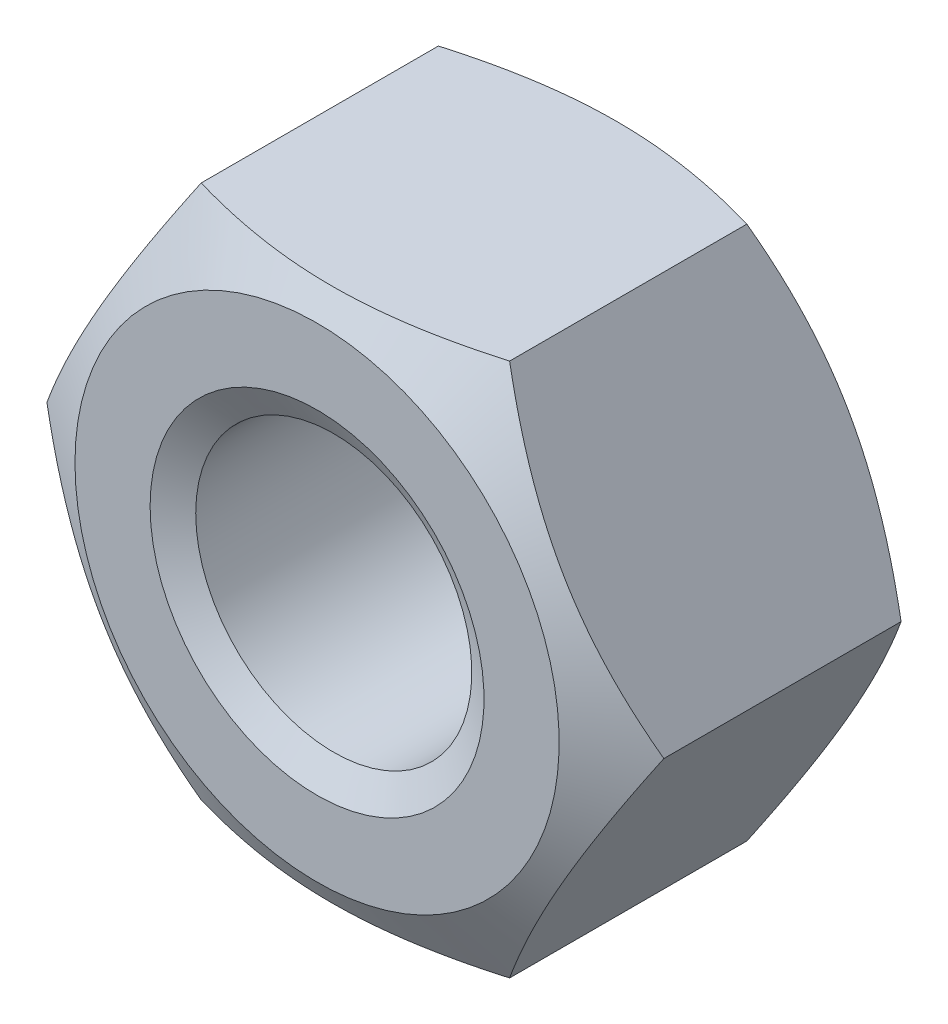
from build123d import *
from OCP.BRepFilletAPI import BRepFilletAPI_MakeChamfer

# Parameters (mm, degrees)
SKETCH1_R        = 2.067
BASENUT_DEPTH    = 4.7
ENDCHAMFER_SIZE  = 0.433
ENDCHAMFER_SIZE2 = 0.249992667


with BuildPart() as part:
    # Sketch1 → BaseNut (new body)
    with BuildSketch(Plane.XY):
        Polygon((4.618802154, 0), (2.309401077, 4), (-2.309401077, 4), (-4.618802154, 0), (-2.309401077, -4), (2.309401077, -4), align=None)
        Circle(SKETCH1_R, mode=Mode.SUBTRACT)
    extrude(amount=-BASENUT_DEPTH)

    # Sketch2 → Double-Chamfer (revolve, cut)
    with BuildSketch(Plane(origin=(0, 0, 0), x_dir=(1, 0, 0), z_dir=(0, 1, 0))):
        Polygon((-4.618802154, 4.7), (-3.625, 4.7), (-4.618802154, 4.126228059), align=None)
        Polygon((-4.618802154, 0.573771941), (-4.618802154, 0), (-3.625, 0), align=None)
    revolve(axis=Axis((0, 0, -3.375940562), (0, 0, 1)), mode=Mode.SUBTRACT)

    # EndChamfer: one chamfer whose edges measure the first distance from different faces: ONE call of the kernel's chamfer builder (chamfer() names one face for all edges)
    endchamfer_edges_1 = [part.edges().sort_by_distance(p)[0] for p in [
        (-2.067, 0, -4.7),
    ]]
    endchamfer_side_1 = [part.faces().sort_by_distance(p)[0] for p in [
        (-2.067, 0, -2.35),
    ]]
    endchamfer_edges_2 = [part.edges().sort_by_distance(p)[0] for p in [
        (-2.067, 0, 0),
    ]]
    endchamfer_side_2 = [part.faces().sort_by_distance(p)[0] for p in [
        (3.522469517, 0, 0),
    ]]
    endchamfer = BRepFilletAPI_MakeChamfer(part.part.solid().wrapped)
    for e in endchamfer_edges_1:
        endchamfer.Add(ENDCHAMFER_SIZE, ENDCHAMFER_SIZE2, e.wrapped, endchamfer_side_1[0].wrapped)  # the first distance lies on this face
    for e in endchamfer_edges_2:
        endchamfer.Add(ENDCHAMFER_SIZE, ENDCHAMFER_SIZE2, e.wrapped, endchamfer_side_2[0].wrapped)  # the first distance lies on this face
    add(Compound.cast(endchamfer.Shape()), mode=Mode.REPLACE)


solid = part.part
